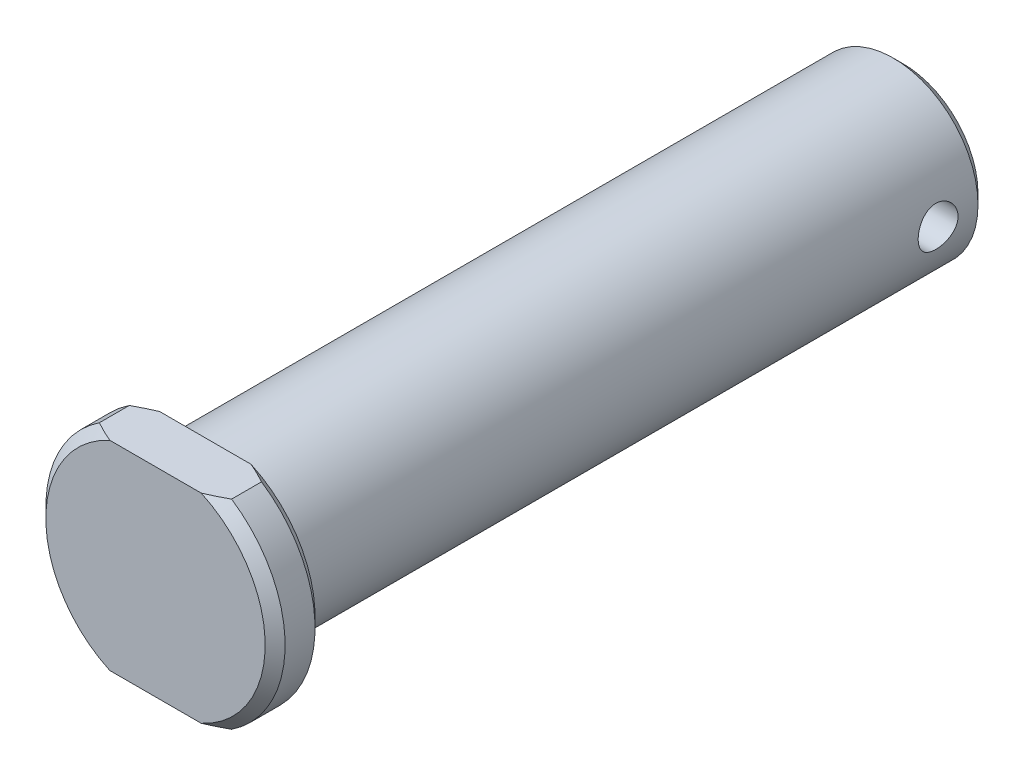
from build123d import *

# Parameters (mm, degrees)
SKETCH2_R          = 2
CUT_EXTRUDE1_DEPTH = 10
SKETCH3_W          = 27.306431106
SKETCH3_H          = 8.074180861
SKETCH3_W_2        = 26.857865503
SKETCH3_H_2        = 8.130251561
CUT_EXTRUDE2_DEPTH = 5
FILLET1_R          = 0.8


with BuildPart() as part:
    # Sketch1 → Revolve1 (revolve)
    with BuildSketch(Plane(origin=(0, 0, 0), x_dir=(0, 0, -1), z_dir=(1, 0, 0)), mode=Mode.PRIVATE) as revolve1_sk:
        Polygon((5, 8.5), (5, 0), (75, 0), (75, 7.5), (74, 8.5), align=None)
        Polygon((4, 12), (5, 11), (5, 0), (0, 0), (0, 11), (1, 12), align=None)
    revolve(revolve1_sk.sketch.rotate(Axis((0, 0, -5), (0, 0, -1)), 90), axis=Axis((0, 0, -5), (0, 0, -1)))

    # Sketch2 → Cut-Extrude1 (cut, symmetric)
    with BuildSketch(Plane(origin=(0, 0, 0), x_dir=(0, 0, -1), z_dir=(1, 0, 0))):
        with Locations((70, 0)):
            Circle(SKETCH2_R)
    extrude(amount=CUT_EXTRUDE1_DEPTH, both=True, mode=Mode.SUBTRACT)

    # Sketch3 → Cut-Extrude2 (cut, symmetric)
    with BuildSketch(Plane.XY):
        with Locations((-0.627385884, 14.037090431)):
            Rectangle(SKETCH3_W, SKETCH3_H)
        with Locations((0.662240226, -14.065125781)):
            Rectangle(SKETCH3_W_2, SKETCH3_H_2)
    extrude(amount=CUT_EXTRUDE2_DEPTH, both=True, mode=Mode.SUBTRACT)

    # Fillet1
    fillet1_edges = [part.edges().sort_by_distance(p)[0] for p in [
        (-8.5, 0, -5),
    ]]
    fillet(fillet1_edges, radius=FILLET1_R)


solid = part.part
